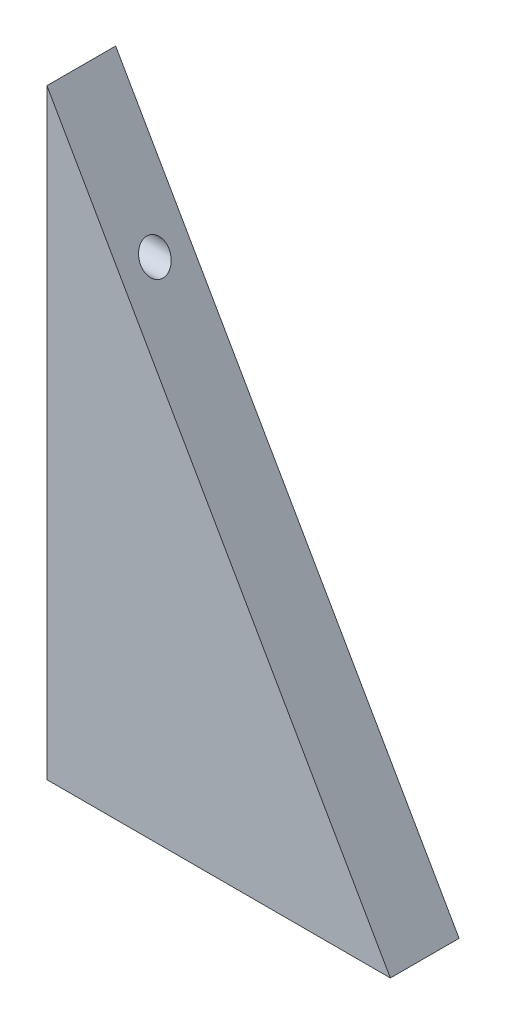
from build123d import *

# Parameters (mm, degrees)
EXTRUDE_1_DEPTH        = 8
HOLE_WIZARD_M4_1_D     = 3.3
HOLE_WIZARD_M4_1_DEPTH = 12
HOLE_WIZARD_M4_1_TIP   = 0.991420021
HOLE_WIZARD_M4_2_D     = 3.3
HOLE_WIZARD_M4_2_DEPTH = 12
HOLE_WIZARD_M4_2_TIP   = 0.991420021


with BuildPart() as part:
    # 草图1 → 凸台-拉伸1 (new body)
    with BuildSketch(Plane.XY):
        Polygon((-20, -35), (20, -35), (-20, 35), align=None)
    extrude(amount=EXTRUDE_1_DEPTH)

    # M4 螺纹孔1
    with Locations(Plane.ZY.offset(20)):
        with Locations((4, -20), (4, 0), (4, 20)):
            Hole(HOLE_WIZARD_M4_1_D / 2, depth=HOLE_WIZARD_M4_1_DEPTH)
            with Locations((0, 0, -(HOLE_WIZARD_M4_1_DEPTH + HOLE_WIZARD_M4_1_TIP / 2))):  # 118° drill point
                Cone(0, HOLE_WIZARD_M4_1_D / 2, HOLE_WIZARD_M4_1_TIP, mode=Mode.SUBTRACT)

    # M4 螺纹孔2
    with Locations(Plane(origin=(0, -35, 0), x_dir=(-1, 0, 0), z_dir=(0, -1, 0))):
        with Locations((-10, -4), (10, -4)):
            Hole(HOLE_WIZARD_M4_2_D / 2, depth=HOLE_WIZARD_M4_2_DEPTH)
            with Locations((0, 0, -(HOLE_WIZARD_M4_2_DEPTH + HOLE_WIZARD_M4_2_TIP / 2))):  # 118° drill point
                Cone(0, HOLE_WIZARD_M4_2_D / 2, HOLE_WIZARD_M4_2_TIP, mode=Mode.SUBTRACT)


solid = part.part
